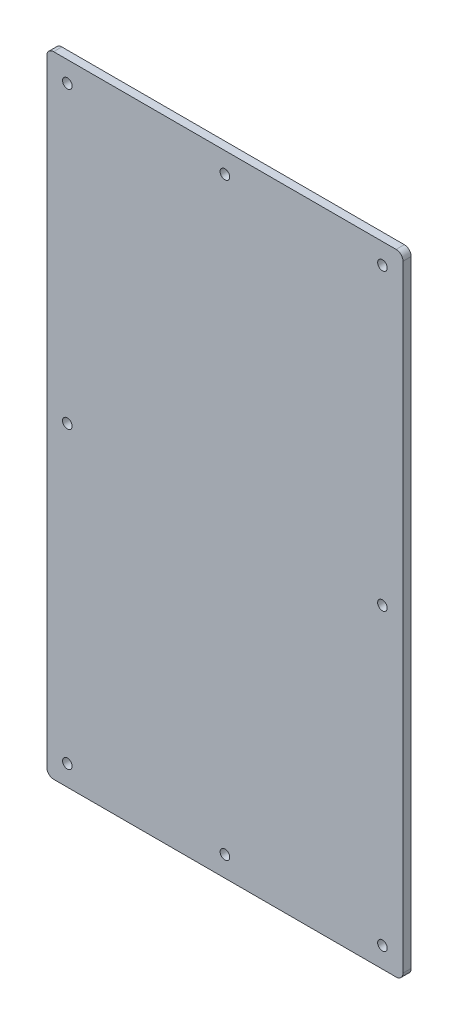
from build123d import *

# Parameters (mm, degrees)
SKETCH_1_W          = 260
SKETCH_1_H          = 460
EXTRUDE_1_DEPTH     = 6
FILLET_1_R          = 5
SKETCH_2_R          = 3.5
CUT_EXTRUDE_1_DEPTH = 529.427856949


with BuildPart() as part:
    # 草图1 → 凸台-拉伸1 (new body)
    with BuildSketch(Plane.XY):
        with Locations((130, -230)):
            Rectangle(SKETCH_1_W, SKETCH_1_H)
    extrude(amount=EXTRUDE_1_DEPTH)

    # 圆角1
    fillet_1_edges = [part.edges().sort_by_distance(p)[0] for p in [
        (0, 0, 3),
        (260, 0, 3),
        (260, -460, 3),
        (0, -460, 3),
    ]]
    fillet(fillet_1_edges, radius=FILLET_1_R)

    # 草图2 → 切除-拉伸1 (cut, through all)
    with BuildSketch(Plane(origin=(0, 0, 0), x_dir=(-1, 0, 0), z_dir=(0, 0, -1))):
        with Locations((-245, -445)):
            Circle(SKETCH_2_R)
        with Locations((-15, -445)):
            Circle(SKETCH_2_R)
        with Locations((-245, -15)):
            Circle(SKETCH_2_R)
        with Locations((-15, -15)):
            Circle(SKETCH_2_R)
        with Locations((-130, -445)):
            Circle(SKETCH_2_R)
        with Locations((-245, -230)):
            Circle(SKETCH_2_R)
        with Locations((-130, -15)):
            Circle(SKETCH_2_R)
        with Locations((-15, -230)):
            Circle(SKETCH_2_R)
    extrude(amount=-CUT_EXTRUDE_1_DEPTH, mode=Mode.SUBTRACT)


solid = part.part
